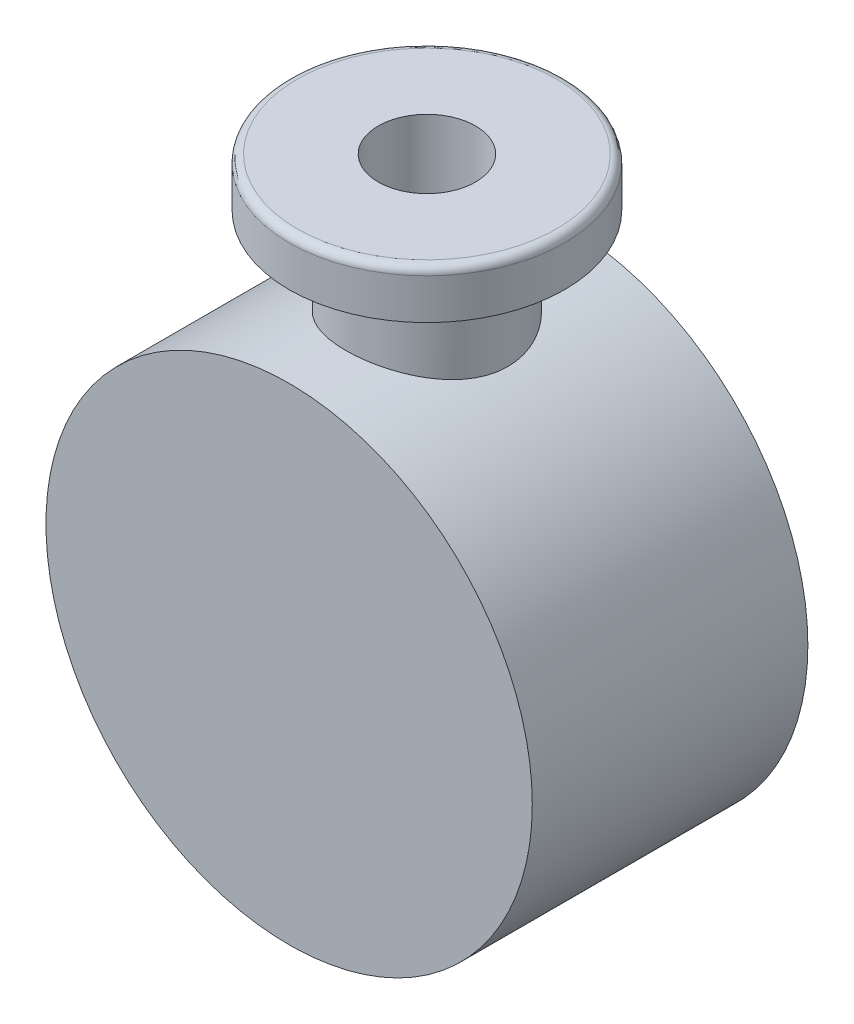
from build123d import *

# Parameters (mm, degrees)
SKETCH1_R                = 15
BOSS_EXTRUDE1_DEPTH      = 8.5
CUT_EXTRUDE1_DEPTH       = 23.852789764
CUT_EXTRUDE1_DEPTH_BACK  = 23.852789764
SKETCH2_R                = 3
BOSS_EXTRUDE2_REACH      = 41.016
BOSS_EXTRUDE2_END_RADIUS = 15
SKETCH3_R                = 5
SKETCH3_R_2              = 3
BOSS_EXTRUDE3_START      = 3
SKETCH4_R                = 8.5
SKETCH4_R_2              = 3
BOSS_EXTRUDE3_DEPTH      = 3
FILLET1_R                = 0.5


with BuildPart() as part:
    # Sketch1 → Boss-Extrude1 (new, symmetric)
    with BuildSketch(Plane.XY):
        Circle(SKETCH1_R)
    extrude(amount=BOSS_EXTRUDE1_DEPTH, both=True)

    # Sketch2 → Cut-Extrude1 (cut, two sides: drawn at the far end of the back side and taken through both)
    with BuildSketch(Plane(origin=(0, 0, 0), x_dir=(1, 0, 0), z_dir=(0, 1, 0)).offset(-CUT_EXTRUDE1_DEPTH_BACK)):
        with Locations(Location((0, 0, 0), (0, 0, 270))):
            Circle(SKETCH2_R)
    extrude(amount=CUT_EXTRUDE1_DEPTH + CUT_EXTRUDE1_DEPTH_BACK, mode=Mode.SUBTRACT)

    # Boss-Extrude2: up to this cylinder (the profile starts outside it)
    boss_extrude2_end = Plane(origin=(0, 0, -4.858579), z_dir=(0, 0, -1)) * Cylinder(BOSS_EXTRUDE2_END_RADIUS, 113.032, mode=Mode.PRIVATE)
    # Sketch3 → Boss-Extrude2 (add, up to the surface)
    with BuildSketch(Plane(origin=(0, 20, 0), x_dir=(1, 0, 0), z_dir=(0, 1, 0)), mode=Mode.PRIVATE) as boss_extrude2_sk1:
        with Locations(Location((0, 0, 0), (0, 0, 270))):
            Circle(SKETCH3_R)
        with Locations(Location((0, 0, 0), (0, 0, 270))):
            Circle(SKETCH3_R_2, mode=Mode.SUBTRACT)
    boss_extrude2_tool1 = extrude(boss_extrude2_sk1.sketch, amount=-BOSS_EXTRUDE2_REACH, mode=Mode.PRIVATE) - boss_extrude2_end
    add(boss_extrude2_tool1.solids().sort_by_distance((0, 20, -4.858579))[0])

    # Sketch4 → Boss-Extrude3 (add)
    with BuildSketch(Plane(origin=(0, 20, 0), x_dir=(1, 0, 0), z_dir=(0, 1, 0)).offset(BOSS_EXTRUDE3_START)):
        with Locations(Location((0, 0, 0), (0, 0, 270))):
            Circle(SKETCH4_R)
        with Locations(Location((0, 0, 0), (0, 0, 270))):
            Circle(SKETCH4_R_2, mode=Mode.SUBTRACT)
    extrude(amount=-BOSS_EXTRUDE3_DEPTH)

    # Fillet1
    fillet1_edges = [part.edges().sort_by_distance(p)[0] for p in [
        (0, 23, -8.5),
    ]]
    fillet(fillet1_edges, radius=FILLET1_R)


solid = part.part
